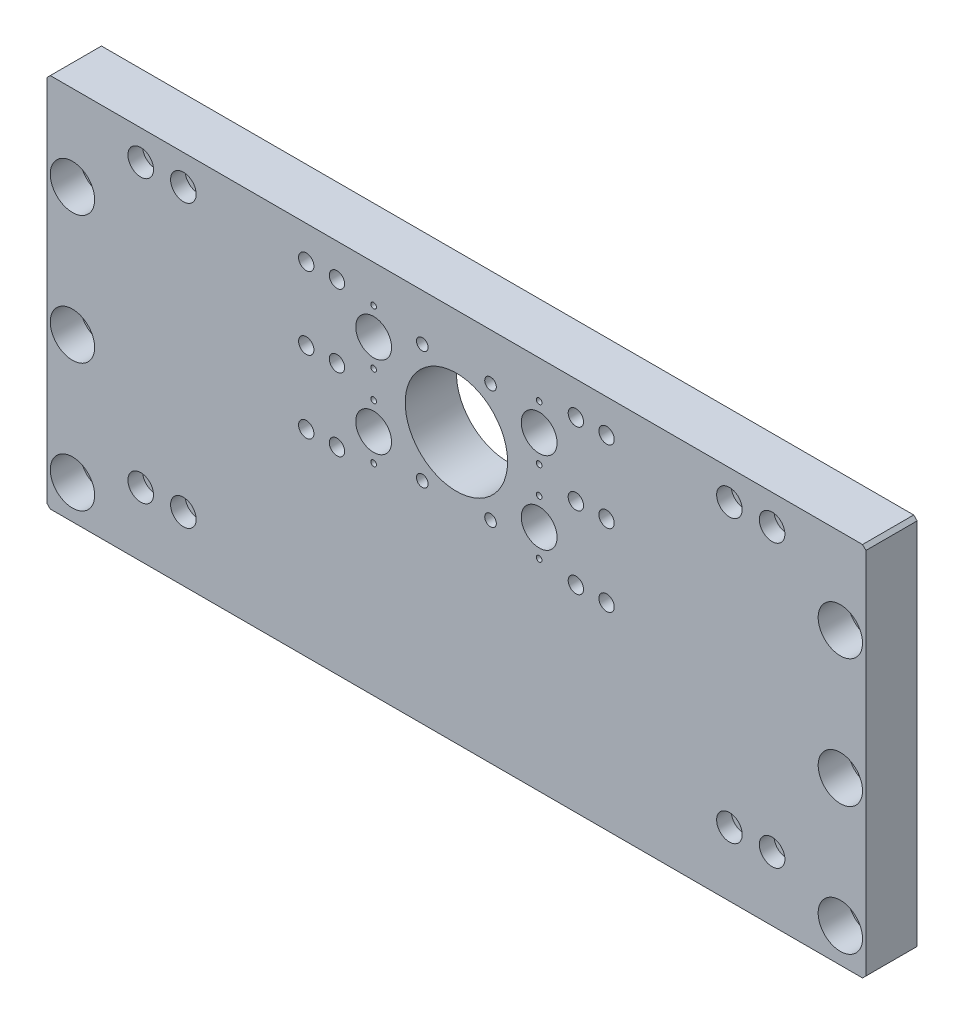
SolidWorks part; units mm, degrees
material "AISI 1045 钢，冷拔"
ref_plane "Front Plane" through (0, 0, 0) normal (0, 0, 1) x (1, 0, 0)
ref_plane "Top Plane" through (0, 0, 0) normal (0, 1, 0) x (1, 0, 0)
ref_plane "Right Plane" through (0, 0, 0) normal (1, 0, 0) x (0, 0, -1)
sketch "Sketch1" plane through (0, 0, 0) normal (0, 0, 1) x (1, 0, 0)
  line L1 (-240, 110) -> (240, 110)
  line L2 (-240, 110) -> (-240, -110)
  line L3 (-240, -110) -> (240, -110)
  line L4 (240, 110) -> (240, -110)
  line L5 (-240, 110) -> (240, -110) construction
  line L6 (-240, -110) -> (240, 110) construction
  point P0 (0, 0)
  dimension "D1" = 220
  dimension "D2" = 480
extrude "Boss-Extrude1" add sketch "Sketch1" along normal mid plane 30
hole_wizard "Hole size per socket head cap screw type2" positions "Sketch3" profile "Sketch2" counterbore size "M16" standard "Gb" end condition through all
sketch "Sketch3" plane through (0, 0, 15) normal (0, 0, 1) x (1, 0, 0)
  line L0 (0, 110) -> (0, -110) construction
  line L1 (240, 110) -> (-240, 110) construction
  line L2 (-240, -110) -> (240, -110) construction
  point P1 (-225, 60)
  point P3 (225, 60)
  point P5 (225, -90)
  point P7 (-225, -90)
  point P21 (-225, -15)
  point P24 (225, -15)
  dimension "D1" = 150
  dimension "D2" = 450
  dimension "D3" = 20
  dimension "D4" = 75
sketch "Sketch2" plane through (-225, 60, 15) normal (1, 0, 0) x (0, -1, 0)
  line L0 (0, 0) -> (0, 30)
  line L1 (0, 30) -> (8.75, 30)
  line L3 (8.75, 30) -> (8.75, 17.5)
  line L4 (8.75, 17.5) -> (13, 17.5)
  line L5 (13, 17.5) -> (13, 0)
  line L7 (13, 0) -> (0, 0)
  line L11 (0, -6.35) -> (0, 107.95) construction
  dimension "通孔孔直径" = 17.5
  dimension "通孔孔深度" = 30
  dimension "柱形沉头孔直径" = 26
  dimension "柱形沉头孔深度" = 17.5
chamfer "Chamfer1" distance 2 angle 45 4 edges at (-240, 110, 0) (-240, -110, 0) (240, -110, 0) (240, 110, 0)
sketch "Sketch4" plane through (0, 0, 15) normal (0, 0, 1) x (1, 0, 0)
  line L0 (238, 110) -> (-238, 110) construction
  circle A0 centre (0, 48) radius 30
  dimension "D1" = 60
  dimension "D2" = 62
extrude "Cut-Extrude1" cut sketch "Sketch4" against normal through all
hole_wizard "M8 Tapped Hole1" positions "Sketch6" profile "Sketch5" tap size "M8" standard "Gb"
sketch "Sketch6" plane through (0, 0, 15) normal (0, 0, 1) x (1, 0, 0)
  line L0 (0, 48) -> (86.6758, 48) construction
  line L2 (0, 48) -> (0, 95.7181) construction
  circle A0 centre (0, 48) radius 40 construction
  point P1 (-20, 82.641)
  point P4 (20, 82.641)
  point P7 (-20, 13.359)
  point P10 (20, 13.359)
  dimension "D2" = 80
  dimension "D1" = 40
sketch "Sketch5" plane through (-20, 82.641, 15) normal (1, 0, 0) x (0, -1, 0)
  line L0 (0, 0) -> (0, 21.7929)
  line L1 (0, 21.7929) -> (3.4, 19.75)
  line L2 (3.4, 19.75) -> (3.4, 0)
  line L5 (3.4, 0) -> (0, 0)
  line L10 (0, 21.7929) -> (-3.4, 19.75) construction
  line L11 (0, -6.35) -> (0, 107.95) construction
  dimension "螺纹孔钻头直径" = 6.8
  dimension "螺纹孔钻头深度" = 19.75
  dimension "导头角度" = 118
cosmetic thread "Cosmetic Thread16" parameters "D1"=16, "D2"=8
cosmetic thread "Cosmetic Thread17" parameters "D1"=16, "D2"=8
cosmetic thread "Cosmetic Thread18" parameters "D1"=16, "D2"=8
cosmetic thread "Cosmetic Thread19" parameters "D1"=16, "D2"=8
hole_wizard "打孔尺寸根据内六角圆柱头螺钉的类型2" positions "Sketch8" profile "Sketch7" counterbore size "M8" standard "GB" end condition through all
sketch "Sketch8" plane through (0, 0, -15) normal (0, 0, -1) x (-1, 0, 0)
  line L0 (-30, 48) -> (30, 48) construction
  line L2 (0, 78) -> (0, 0) construction
  circle A0 centre (0, 48) radius 30 construction
  point P1 (-88, 90.5)
  point P3 (-70, 90.5)
  point P5 (-70, 48)
  point P7 (-88, 48)
  point P9 (-88, 5.5)
  point P11 (-70, 5.5)
  point P15 (70, 90.5)
  point P17 (88, 90.5)
  point P19 (70, 48)
  point P21 (88, 48)
  point P23 (70, 5.5)
  point P25 (88, 5.5)
  dimension "D1" = 18
  dimension "D2" = 18
  dimension "D3" = 140
  dimension "D4" = 85
sketch "Sketch7" plane through (88, 90.5, -15) normal (1, 0, 0) x (0, 1, 0)
  line L0 (0, 0) -> (0, 30)
  line L1 (0, 30) -> (4.5, 30)
  line L3 (4.5, 30) -> (4.5, 9)
  line L4 (4.5, 9) -> (7.5, 9)
  line L5 (7.5, 9) -> (7.5, 0)
  line L7 (7.5, 0) -> (0, 0)
  line L11 (0, -6.35) -> (0, 107.95) construction
  dimension "通孔孔直径" = 9
  dimension "通孔孔深度" = 30
  dimension "柱形沉头孔直径" = 15
  dimension "柱形沉头孔深度" = 9
sketch "Sketch9" plane through (0, 0, 15) normal (0, 0, 1) x (1, 0, 0)
  line L0 (0, 78) -> (0, 18) construction
  line L1 (-30, 48) -> (30, 48) construction
  circle A0 centre (-48.5, 72) radius 10.5
  circle A1 centre (-48.5, 24) radius 10.5
  circle A2 centre (48.5, 24) radius 10.5
  circle A3 centre (48.5, 72) radius 10.5
  circle A4 centre (0, 48) radius 30 construction
  dimension "D1" = 21
  dimension "D2" = 48
  dimension "D3" = 97
extrude "Cut-Extrude2" cut sketch "Sketch9" against normal through all
hole_wizard "M4 Tapped Hole1" positions "Sketch11" profile "Sketch10" tap size "M4" standard "GB"
sketch "Sketch11" plane through (0, 0, 15) normal (0, 0, 1) x (1, 0, 0)
  line L0 (48.5, 82.5) -> (48.5, 13.5) construction
  line L2 (38, 72) -> (59, 72) construction
  line L4 (38, 24) -> (59, 24) construction
  circle A0 centre (48.5, 72) radius 10.5 construction
  circle A1 centre (48.5, 24) radius 10.5 construction
  point P1 (48.5, 88)
  point P3 (48.5, 56)
  point P5 (48.5, 40)
  point P7 (48.5, 8)
  dimension "D1" = 32
  dimension "D2" = 32
sketch "Sketch10" plane through (48.5, 88, 15) normal (1, 0, 0) x (0, -1, 0)
  line L0 (0, 0) -> (0, 11.0914)
  line L1 (0, 11.0914) -> (1.65, 10.1)
  line L2 (1.65, 10.1) -> (1.65, 0)
  line L5 (1.65, 0) -> (0, 0)
  line L10 (0, 11.0914) -> (-1.65, 10.1) construction
  line L11 (0, -6.35) -> (0, 107.95) construction
  dimension "螺纹孔钻头直径" = 3.3
  dimension "螺纹孔钻头深度" = 10.1
  dimension "导头角度" = 118
cosmetic thread "Cosmetic Thread7" parameters "D1"=8, "D2"=4
cosmetic thread "Cosmetic Thread8" parameters "D1"=8, "D2"=4
cosmetic thread "Cosmetic Thread9" parameters "D1"=8, "D2"=4
cosmetic thread "Cosmetic Thread13" parameters "D1"=8, "D2"=4
mirror "Mirror1" about plane through (0, 0, 0) normal (1, 0, 0) of "M4 Tapped Hole1"
hole_wizard "CBORE for M8 Hex Socket Head Cap Screw1" positions "Sketch13" profile "Sketch12" counterbore size "M8" standard "Iso" end condition through all
sketch "Sketch13" plane through (0, 0, 15) normal (0, 0, 1) x (1, 0, 0)
  point P0 (-185, -72.5)
  point P3 (-160, -72.5)
  point P6 (-185, 92.5)
  point P9 (-160, 92.5)
  point P12 (185, 92.5)
  point P15 (160, 92.5)
  point P18 (185, -72.5)
  point P21 (160, -72.5)
sketch "Sketch12" plane through (-185, -72.5, 15) normal (1, 0, 0) x (0, -1, 0)
  line L0 (0, 0) -> (0, 30)
  line L1 (0, 30) -> (4.5, 30)
  line L3 (4.5, 30) -> (4.5, 8.6)
  line L4 (4.5, 8.6) -> (7.5, 8.6)
  line L5 (7.5, 8.6) -> (7.5, 0)
  line L7 (7.5, 0) -> (0, 0)
  line L11 (0, -6.35) -> (0, 107.95) construction
  dimension "通孔孔直径" = 9
  dimension "通孔孔深度" = 30
  dimension "柱形沉头孔直径" = 15
  dimension "柱形沉头孔深度" = 8.6
